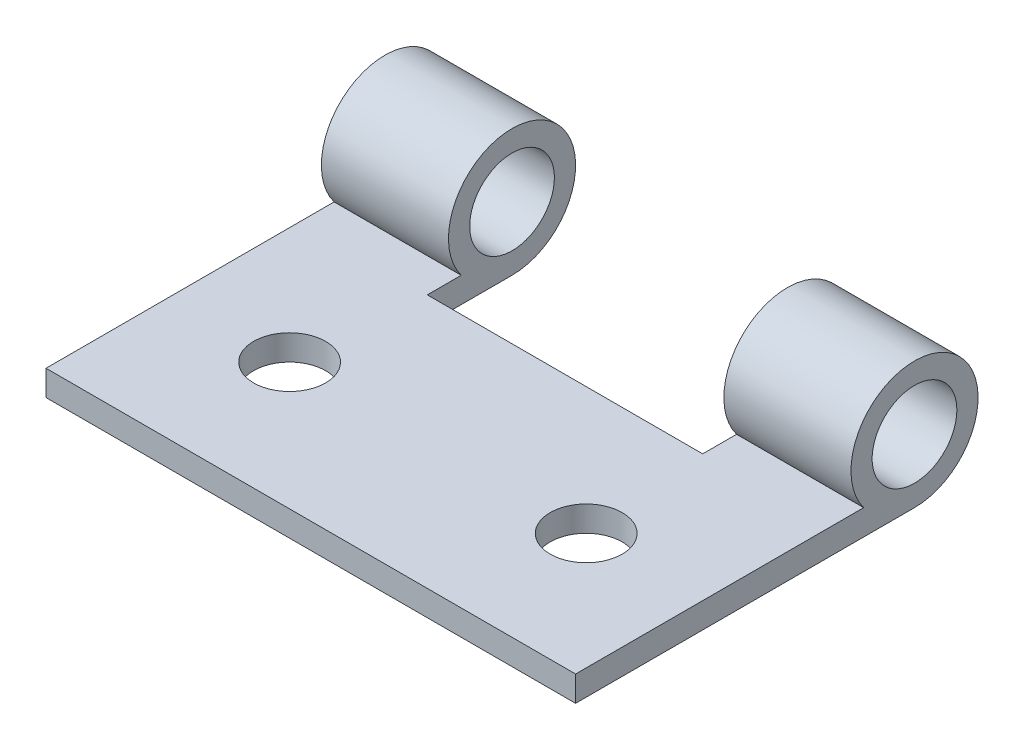
SolidWorks part; units mm, degrees
material "AISI 304"
ref_plane "前视基准面" through (0, 0, 0) normal (0, 0, 1) x (1, 0, 0)
ref_plane "上视基准面" through (0, 0, 0) normal (0, 1, 0) x (1, 0, 0)
ref_plane "右视基准面" through (0, 0, 0) normal (1, 0, 0) x (0, 0, -1)
sketch "草图1" plane through (0, 0, 0) normal (1, 0, 0) x (0, 0, -1)
  line L0 (0, -3) -> (-16, -3)
  line L1 (-16, -3) -> (-16, -1.8)
  line L2 (-16, -1.8) -> (-2.4, -1.8)
  arc A0 (0, -3) -> (-2.4, -1.8) centre (0, 0) ccw
  circle A1 centre (0, 0) radius 2
  dimension "D1" = 3
  dimension "D4" = 4
  dimension "D2" = 16
  dimension "D3" = 1.2
extrude "凸台-拉伸1" add sketch "草图1" along normal mid plane 25
sketch "草图2" plane through (0, -1.8, 0) normal (0, 1, 0) x (1, 0, 0)
  line L0 (-7, -10) -> (7, -10) construction
  line L1 (0, 0) -> (0, -16) construction
  line L2 (12.5, -16) -> (-12.5, -16) construction
  circle A0 centre (-7, -10) radius 1.7
  circle A1 centre (7, -10) radius 1.7
  dimension "D1" = 10
  dimension "D3" = 3.4
  dimension "D2" = 14
extrude "切除-拉伸1" cut sketch "草图2" against normal through all
sketch "草图3" plane through (0, 0, 0) normal (1, 0, 0) x (0, 0, -1)
  line L0 (-16, -3) -> (0, -3) construction
  line L1 (-2.4, -1.8) -> (-16, -1.8) construction
  line L2 (-4, -3) -> (0, -3)
  line L3 (-2.4, -1.8) -> (-4, -1.8)
  line L4 (-4, -1.8) -> (-4, -3)
  arc A0 (0, -3) -> (-2.4, -1.8) centre (0, 0) ccw construction
  arc A1 (0, -3) -> (-2.4, -1.8) centre (0, 0) ccw
  dimension "D1" = 4
extrude "切除-拉伸2" cut sketch "草图3" against normal mid plane 13
